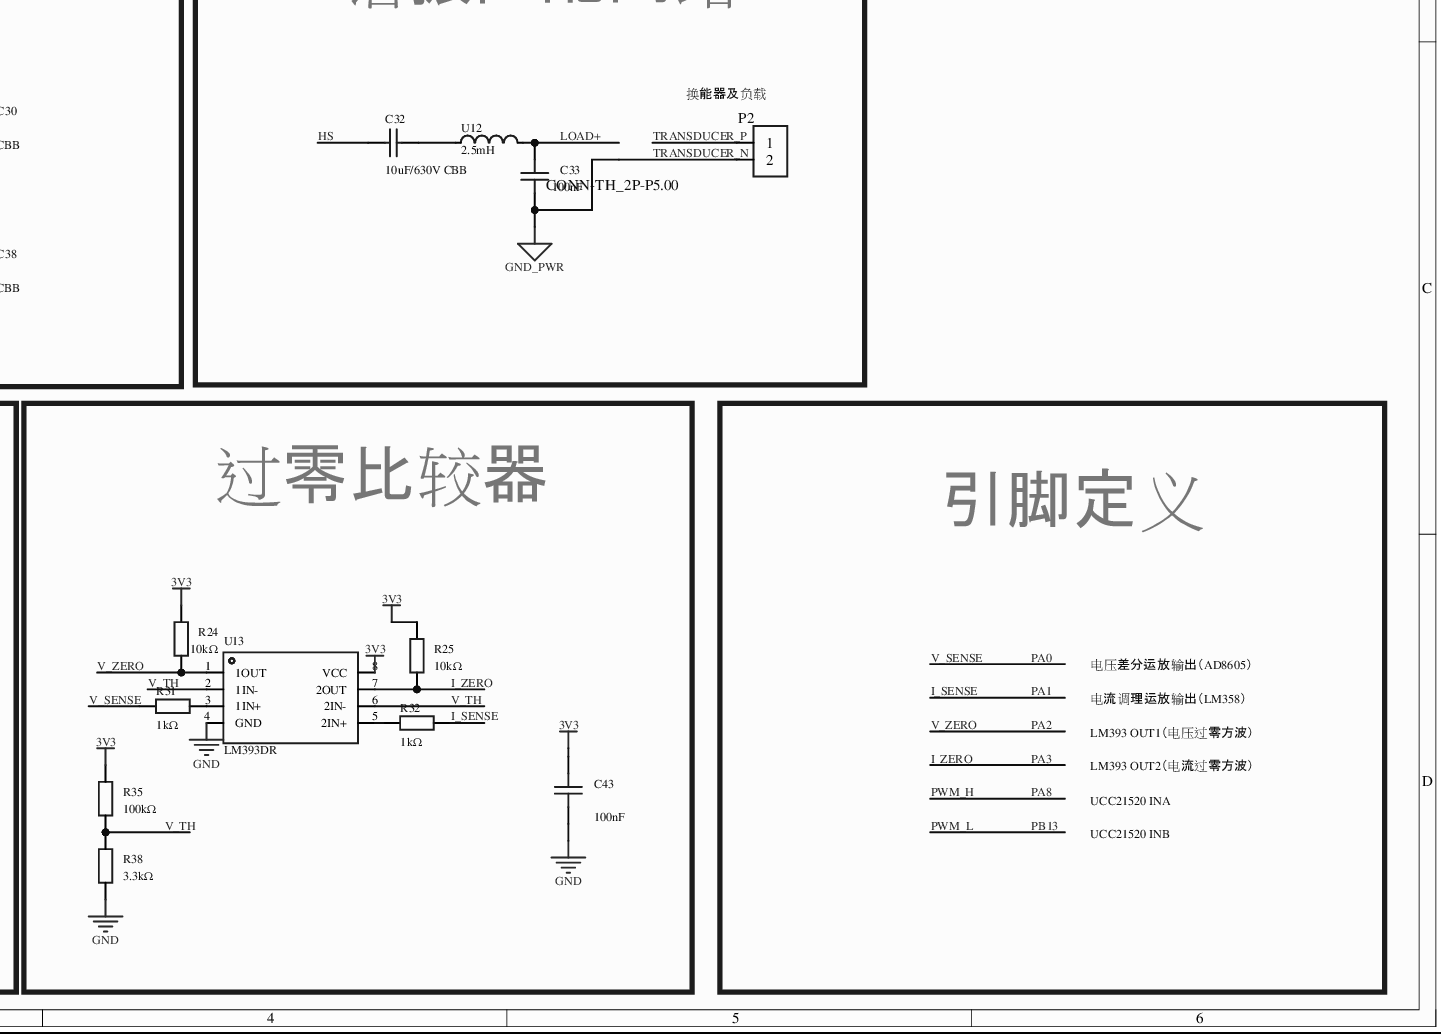
[diagram p0: MISC51807-3.schdoc, bottom right]
# Altium project MISC51807-2.PrjPcb (part 2 of 2)
## Sheet MISC51807-3.schdoc (continued)
### Library data of the parts (continued)
D2 = BYV26C: 二极管配置:独立式;正向压降(Vf):2.5V@1A;直流反向耐压(Vr):600V;整流电流:1A;反向恢复时间(Trr):30ns;; Manufacturer: LGE(鲁光); Symbol: BYV26C_C2903806; AddInBom: yes; ModelId: 24566a456941402eb024cf45acdcf6880819f05c4eef4c71ace90d822a990e87; ModelTransform: 385.826,102.71814,0,0,0,0,0,0,-196.85; Diode Configuration: 独立式; Voltage - DC Reverse(Vr): 600V; Current - Rectified: 1A; Reverse Leakage Current (Ir): 5uA@600V; Reverse Recovery Time (trr): 30ns; Operating Junction Temperature Range: -55℃~+150℃@(Tj); Non-Repetitive Peak Forward Surge Current: 30A; Device: BYV26C; LCSC Part Name: 耐压:600V 电流:1A 反向恢复时间：30ns; SupplierPart: C2903806; ManufacturerPart: BYV26C; Supplier Footprint: DO-41; JLCPCB Part Class: Extended Part; Datasheet: https://item.szlcsc.com/datasheet/BYV26C/3160571.html; Supplier: LCSC; ConvertToPcb: yes; FootprintName: DO-41_BD2.6-L5.1-P9.00-D0.8-RD; ModelName: DO-41_BD2.6-L5.1-P9.00-D0.8-RD; Voltage - Forward(Vf@If): 2.5V@1A
D3 = SR5100_C784810: 二极管配置:独立式;正向压降(Vf):850mV@5A;直流反向耐压(Vr):100V;整流电流:5A;; Manufacturer: FUXINSEMI(富芯森美); 3D Model: f76203e12ec84be0b89e1bb5efd9c700; 3D Model Transform: 582.676,208.5295,0,0,0,0,0,0,-137.795; Diode Configuration: 独立式; Voltage - DC Reverse(Vr): 100V; Current - Rectified: 5A; AddInBom: yes; ModelName: DO-201AD_D5.3-L8.4-P13.6; Symbol: SR5100_C784810; Device: SR5100_C784810; LCSC Part Name: 电压:100V 电流:5A; Supplier Part: C784810; Manufacturer Part: SR5100; Supplier Footprint: DO-27; JLCPCB Part Class: 扩展库; Datasheet: https://atta.szlcsc.com/upload/public/pdf/source/20200917/C784810_F194D3227990C9BBD8D528E4C494EB0B.pdf; Supplier: LCSC; Voltage - Forward(Vf@If): 850mV@5A; Reverse Leakage Current (Ir): -; ConvertToPcb: yes; FootprintName: DO-201AD_BD5.3-L8.4-P12.50-D1.4-RD
D4 D5 = 1N5819_C110032: 正向压降(Vf):550mV@1A;直流反向耐压(Vr):40V;整流电流:1A;; Manufacturer: ST(意法半导体); 3D Model: 6de1e9b71a0d4751b4e9df530304c1a3; 3D Model Transform: 374.015,94.428,0,180,0,0,0,0,-137.795; Reverse Voltage (Vr): 40V; Rectified Current: 1A; Reverse Leakage Current (Ir): 500uA@40V; AddInBom: yes; ModelName: DO-41_D2.4-L4.7-P8.70; Symbol: 1N5819; Device: 1N5819_C110032; LCSC Part Name: 电压:40V 电流:1A; Supplier Part: C110032; Manufacturer Part: 1N5819; Supplier Footprint: DO-41; JLCPCB Part Class: 扩展库; Datasheet: https://atta.szlcsc.com/upload/public/pdf/source/20170428/1493376792224.pdf; Supplier: LCSC; Forward Voltage (Vf@If): 550mV@1A; ConvertToPcb: yes; FootprintName: DO-41_BD2.4-L4.7-P8.70-D0.9-FD
D6 D7 = BZT52C3V3S_C19077437: 二极管配置:独立式;稳压值(标称值):3.3V;稳压值(范围):3.1V~3.5V;耗散功率(Pd):200mW;; Manufacturer: R+O(宏嘉诚); AddInBom: yes; ModelId: 8f7582057468434a979d3a4d6e318d8a0819f05c4eef4c71ace90d822a990e87; ModelTransform: 100.394,49.2125,0,0,0,0,0,0,0; Diode Configuration: 独立式; Zener Voltage(Nom): 3.3V; Reverse Leakage Current (Ir): 5uA@1.0V; Pd - Power Dissipation: 200mW; Impedance(Zzt): 95Ω; Impedance(Zzk): 600Ω; Operating Junction Temperature Range: -55℃~+150℃; Symbol: BZT52C3V3S_C19077437; Device: BZT52C3V3S_C19077437; LCSC Part Name: 表面贴装齐纳二极管; SupplierPart: C19077437; ManufacturerPart: BZT52C3V3S; Supplier Footprint: SOD-323; JLCPCB Part Class: Extended Part; Datasheet: https://item.szlcsc.com/datasheet/BZT52C3V3S/20275522.html; Supplier: LCSC; ConvertToPcb: yes; FootprintName: SOD-323_L1.7-W1.3-LS2.6-RD; ModelName: SOD-323_L1.7-W1.3-LS2.6-RD; Zener Voltage(Range): 3.1V~3.5V
F1 = MTS1315A: 类型:方形保险丝;额定电流:3.15A;额定电压:250V;分断能力:35A@250VAC;; Manufacturer: Reomax(瑞迈); AddInBom: yes; ModelId: 221481fd52dd4abc8b2b4285dcb66f990819f05c4eef4c71ace90d822a990e87; ModelTransform: 330.708,157.48,0,0,0,0,0,0,-157.48; Type: 方形保险丝; Current Rating: 3.15A; Voltage Rating (DC): 250V; Melting I2t: 64; Pitch: 5.08mm; Symbol: MTS1315A; Device: MTS1315A; LCSC Part Name: 方形直插 慢断 250V 3.15A 保险丝; SupplierPart: C2762408; ManufacturerPart: MTS1315A; Supplier Footprint: 插件,P=5.08mm; JLCPCB Part Class: Extended Part; Datasheet: https://item.szlcsc.com/datasheet/MTS1315A/2889364.html; Supplier: LCSC; ConvertToPcb: yes; FootprintName: FUSE-TH_L8.4-W4.0-P5.08-D0.6; ModelName: FUSE-TH_L8.4-W4.0-P5.08-D0.6; Operating Temperature: -55℃~+125℃; Interrupt Rating: 35A@250VAC; Length: 8.4mm; Width: 4mm; Height: 7.2mm
H1 = PZ254V-11-01P: 插针结构:1x1P;间距:2.54mm;行距:-;圆针/方针:方针;安装方式:直插;排数:单排;总PIN位数:1P;额定电流:-;额定电压:-;配合针长度:6mm;塑高:2.5mm;端接针长度:3mm;触头材质:黄铜;触头镀层:-;工作温度:-40℃~+105℃;颜色:黑色;; Manufacturer: XFCN(兴飞); 3D Model: efa57846279b44bfa0a28253a2c74e33; 3D Model Transform: 100,100,0,0,0,0,0,0,-118.11; Pin Structure: 1x1P; Pitch: 2.54mm; Circluar Pins/Square Pins: 方针; AddInBom: yes; ModelName: HDR2.54-M-LI-1X1P; Symbol: PZ254V-11-01P; Device: PZ254V-11-01P; LCSC Part Name: 1x1P 间距:2.54mm 方针 直插; Supplier Part: C492400; Manufacturer Part: PZ254V-11-01P; Supplier Footprint: 插件,P=2.54mm; JLCPCB Part Class: 扩展库; Datasheet: https://atta.szlcsc.com/upload/public/pdf/source/20200309/C492400_46876A5B545F5AE6B8D4A09C46E276E8.pdf; Supplier: LCSC; Row Spacing: -; Mounting Type: 直插; Number of Rows: 单排; Number of Pins: 1P; Current Rating: -; Voltage Rating (Max): -; Length of Mating Pin: 6mm; Insulation Height: 2.5mm; Length of End Connection Pin: 3mm; Contact Material: 黄铜; Contact Plating: -; Operating Temperature: -40℃~+105℃; Color: 黑色; ConvertToPcb: yes; FootprintName: HDR-TH_1P-P2.54-V-M
J1 J2 = 2.54-1*20P直针: 排数:单排;总PIN位数:20;间距:2.54mm;插针结构:1x20P;行距:-;安装类型:直插;圆针/方针:方针;额定电流:3A;额定电压:-;配合针长度:-;塑高:-;端接针长度:-;触头材质:黄铜;触头镀层:-;工作温度范围:-40~+105;颜色:黑色;; Manufacturer: BOOMELE(博穆精密); Symbol: Header-Male-2.54_1x20; 3D Model: f68709be121d406db68b06f32a595389; 3D Model Transform: 1999.996,100,0,0,0,0,0,2.48,-118.11; Pitch: 2.54mm; Pin Structure: 1x20P; Circluar Pins/Square Pins: 方针; Current Rating (Max): 3A; AddInBom: yes; ModelName: HDR-M-2.54_1x20; Device: 2.54-1*20P直针; Operating Temperature Range: -40~+105; LCSC Part Name: 2.54mm 1x20P 直插 方针; Supplier Part: C50981; Manufacturer Part: 2.54-1*20P直针; Supplier Footprint: 插件,P=2.54mm; JLCPCB Part Class: Extended Part; Datasheet: https://atta.szlcsc.com/upload/public/pdf/source/20151109/1457707571495.pdf; Supplier: LCSC; Number of Rows: 单排; Number of Pins: 20; Row Spacing: -; Mounting Type: 直插; Voltage Rating (Max): -; Length of Mating Pin: -; Insulation Height: -; Length of End Connection Pin: -; Contact Material: 黄铜; Contact Plating: -; Color: 黑色; ConvertToPcb: yes; FootprintName: HDR-TH_20P-P2.54-V-M-1
L1 = PDMCAT16128-103ML: 通道数:2;电感@频率:10mH@1kHz;直流电阻(DCR):75mΩ;; Manufacturer: PROD(谱罗德); AddInBom: yes; ModelId: 59532b68e412455698164cb9480e4efc0819f05c4eef4c71ace90d822a990e87; ModelTransform: 787.4,444.881,0,0,0,0,-0.591,0,-196.85; Number of Lines: 2; Voltage Withstand: 600V@AC,3secs; Current Rating: 3A; Voltage Rating - DC: 600V; DC Resistance(DCR): 75mΩ; Symbol: PDMCAT16128-103ML; Device: PDMCAT16128-103ML; LCSC Part Name: 两路 插件共模滤波器; SupplierPart: C2762380; ManufacturerPart: PDMCAT16128-103ML; Supplier Footprint: 插件,20x18mm; JLCPCB Part Class: Extended Part; Datasheet: https://atta.szlcsc.com/upload/public/pdf/source/20210322/C2762380_4CF5A8B18369ADCA8640E34A9EF957E4.pdf; Supplier: LCSC; ConvertToPcb: yes; FootprintName: IND-TH_4P-L20.0-W12.0-P6.00-LS10.0-BL; ModelName: IND-TH_4P-L20.0-W12.0-P6.00-LS10.0-BL; Inductance @ Frequency: 10mH@1kHz; Voltage Rating (AC): 600V; Operating Temperature: -25℃~+85℃
L2 = SLP0810R-102MTT: 电感值:1mH;精度:±20%;额定电流:500mA;类型:工字电感;; Manufacturer: Sunltech(顺磁); AddInBom: yes; ModelId: f824c3cd5f0947e0ad34b4cb921321ba0819f05c4eef4c71ace90d822a990e87; ModelName: IND-TH_BD8.5-H8.3-P5.00-D0.6; ModelTransform: 334.645,334.645,0,0,0,0,-0.005,0,-196.85; Tolerance: ±20%; Current Rating: 500mA; DC Resistance(DCR): 1.8Ω; Type: 工字电感; Symbol: SLP0810R-102MTT; Device: SLP0810R-102MTT; LCSC Part Name: 1mH ±20%; SupplierPart: C364093; ManufacturerPart: SLP0810R-102MTT; Supplier Footprint: 插件,D8.5xL12mm; JLCPCB Part Class: Extended Part; Datasheet: https://item.szlcsc.com/datasheet/SLP0810R-102MTT/338381.html; Supplier: LCSC; ConvertToPcb: yes; FootprintName: IND-TH_BD8.5-P5.00-D0.6; Value: 1mH
OLED1 = 0.96OLED模块_4P: 3D Model: 79c000fdb68d45a296c2e9bedf4f9055; 3D Model Transform: 1393.69792,1318.895,0,0,0,0,0,-560.079,-137.795; ConvertToPcb: yes; Symbol: 0.96OLED模块_4P; Device: 0.96OLED模块_4P; Supplier Footprint: 插件; AddInBom: yes; FootprintName: 0.96OLED_4P; ModelName: 0.96OLED_4P
P1 P2 = CONN-TH_2P-P5.00: Add into BOM: yes; 3D Model: 82ed0e208d9a4cc2ac854dcad4b56f25; Symbol: CONN-TH_2P-P5.00; Device: CONN-TH_2P-P5.00; Convert to PCB: yes; Supplier: LCSC; FootprintName: CONN-TH_2P-P5.00; ModelName: CONN-TH_2P-P5.00
Q1 Q2 = IRF840_C2980294: 数量:1个N沟道;漏源电压(Vdss):500V;连续漏极电流(Id):8A;导通电阻(RDS(on)):730mΩ@10V;耗散功率(Pd):134W;阈值电压(Vgs(th)):3V@250uA;; Manufacturer: minos(迈诺斯); AddInBom: yes; ModelId: 0369bc25c9bd44718af72a1d71ffd3cd0819f05c4eef4c71ace90d822a990e87; ModelTransform: 401.574,177.204,0,0,0,0,0,24.606,-196.85; Number: 1个N沟道; Drain to Source Voltage: 500V; Current - Continuous Drain(Id): 8A; Pd - Power Dissipation: 134W; Gate Charge(Qg): 25nC@10V; Input Capacitance(Ciss): 1.57nF; Reverse Transfer Capacitance (Crss@Vds): 20pF; Type: N沟道; Output Capacitance(Coss): 195pF; Symbol: IRF840_C2980294; Device: IRF840_C2980294; LCSC Part Name: N沟道,电流:8A,耐压:500V; SupplierPart: C2980294; ManufacturerPart: IRF840; Supplier Footprint: TO-220; JLCPCB Part Class: Extended Part; Datasheet: https://item.szlcsc.com/datasheet/IRF840/3401452.html; Supplier: LCSC; ConvertToPcb: yes; FootprintName: TO-220-3_L10.2-W4.5-P2.54-L-1; ModelName: TO-220-3_L10.2-W4.5-P2.54-L-1; RDS(on): 730mΩ@10V; Gate Threshold Voltage (Vgs(th)): 3V@250uA; Operating Temperature: -
R1 = 0603WAF6201T5E: 电阻类型:厚膜电阻;阻值:6.2kΩ;精度:±1%;功率:100mW;工作电压:75V;温度系数:±100ppm/℃;; Manufacturer: UNI-ROYAL(厚声); AddInBom: yes; ModelId: fc143cca1e79419f9cd78b61e9279f080819f05c4eef4c71ace90d822a990e87; ModelTransform: 31.8897,63.7794,0,90,0,0,0,0,0; Tolerance: ±1%; Power(Watts): 100mW; Voltage-Supply(Max): 75V; Symbol: 0603WAF6201T5E; Device: 0603WAF6201T5E; LCSC Part Name: 6.2kΩ ±1% 100mW 厚膜电阻; SupplierPart: C4260; ManufacturerPart: 0603WAF6201T5E; Supplier Footprint: 0603; JLCPCB Part Class: Basic Part; Datasheet: https://item.szlcsc.com/datasheet/0603WAF6201T5E/4667.html; Supplier: LCSC; ConvertToPcb: yes; FootprintName: R0603; ModelName: R0603; Type: 厚膜电阻; Value: 6.2kΩ; Temperature Coefficient: ±100ppm/℃; Operating Temperature: -55℃~+155℃
R2 = 0603WAF2002T5E: 电阻类型:厚膜电阻;阻值:20kΩ;精度:±1%;功率:100mW;工作电压:75V;温度系数:±100ppm/℃;; Manufacturer: UNI-ROYAL(厚声); AddInBom: yes; ModelId: fc143cca1e79419f9cd78b61e9279f080819f05c4eef4c71ace90d822a990e87; ModelTransform: 31.8897,63.7794,0,90,0,0,0,0,0; Tolerance: ±1%; Power(Watts): 100mW; Voltage-Supply(Max): 75V; Symbol: 0603WAF2002T5E; Device: 0603WAF2002T5E; LCSC Part Name: 20kΩ ±1% 100mW 厚膜电阻; SupplierPart: C4184; ManufacturerPart: 0603WAF2002T5E; Supplier Footprint: 0603; JLCPCB Part Class: Basic Part; Datasheet: https://item.szlcsc.com/datasheet/0603WAF2002T5E/4591.html; Supplier: LCSC; ConvertToPcb: yes; FootprintName: R0603; ModelName: R0603; Type: 厚膜电阻; Value: 20kΩ; Temperature Coefficient: ±100ppm/℃; Operating Temperature: -55℃~+155℃
R3 = 14D471K_C49069733: 压敏电压:470V;钳位电压:775V;工作电压(DC):385V;工作电压(AC):300V;; Manufacturer: R+O(宏嘉诚); AddInBom: yes; ModelId: 3cca2a1a348a43d9bb99ecdc91f351c80819f05c4eef4c71ace90d822a990e87; ModelName: RES-TH_L15.5-W5.6-H18.5-P7.50-D0.8-S1.90; ModelTransform: 610.19083,220.472,0,0,0,0,0,0,-196.85; Varistor Voltage: 470V; Clamping Voltage: 775V; Maximum DC Volts: 385V; Maximum AC Volts: 300V; Peak Current: 4.5kA; Energy: 148J; Rated Wattage: 600mW; Symbol: 14D471K_C49069733; Device: 14D471K_C49069733; LCSC Part Name: 775V 148J; SupplierPart: C49069733; ManufacturerPart: 14D471K; Supplier Footprint: 插件,P=7.5mm; JLCPCB Part Class: Extended Part; Datasheet: https://item.szlcsc.com/datasheet/14D471K/51445299.html; Supplier: LCSC; ConvertToPcb: yes; FootprintName: RES-TH_L15.5-W5.6-P7.50-D0.8-S1.90; Value: 420pF@1kHz
R4 = FMP200JR-52-220K: 电阻类型:金属膜电阻;阻值:220kΩ;精度:±5%;功率:2W;温度系数:±100ppm/℃;; Manufacturer: YAGEO(国巨); AddInBom: yes; ModelId: 8ab905774ec2447d84fda7276baf35870819f05c4eef4c71ace90d822a990e87; ModelTransform: 543.306,153.44056,0,0,0,0,0,0,-196.85; Tolerance: ±5%; Power(Watts): 2W; Symbol: FMP200JR-52-220K; Device: FMP200JR-52-220K; LCSC Part Name: 金属膜电阻 220kΩ ±5% 2W; SupplierPart: C1759543; ManufacturerPart: FMP200JR-52-220K; Supplier Footprint: 插件,D3.9xL9mm; JLCPCB Part Class: Extended Part; Datasheet: https://item.szlcsc.com/datasheet/FMP200JR-52-220K/1850325.html; Supplier: LCSC; ConvertToPcb: yes; FootprintName: RES-TH_BD3.9-L9.0-P13.00-D0.8; ModelName: RES-TH_BD3.9-L9.0-P13.00-D0.8; Type: 金属膜电阻; Value: 220kΩ; Temperature Coefficient: ±100ppm/℃; Operating Temperature: -55℃~+155℃
R6 R7 = 0603WAF1002T5E: 电阻类型:厚膜电阻;阻值:10kΩ;精度:±1%;功率:100mW;温度系数:±100ppm/;最大工作电压:75V;工作温度范围:-55~+155;; Manufacturer: UNI-ROYAL(厚声); 3D Model: 3281a289d46d4bb1877be1eabd090e13; 3D Model Transform: 62.992,31.496,0,0,0,0,0,0,0; Tolerance: ±1%; Power(Watts): 100mW; Overload Voltage (Max): 75V; AddInBom: yes; ModelName: R0603_L1.6-W0.8-H0.8; Symbol: 0603WAF1002T5E; Device: 0603WAF1002T5E; Value: 10kΩ; Temperature Coefficient: ±100ppm/; Operating Temperature Range: -55~+155; LCSC Part Name: 10kΩ ±1% 100mW; Supplier Part: C25804; Manufacturer Part: 0603WAF1002T5E; Supplier Footprint: 0603; JLCPCB Part Class: Basic Part; Datasheet: https://atta.szlcsc.com/upload/public/pdf/source/20200306/C422600_1E6D84923E4A46A82E41ADD87F860B5C.pdf; Supplier: LCSC; Type: 厚膜电阻; ConvertToPcb: yes; FootprintName: R0603_1
R8 R9 = 0603WAF4701T5E: 电阻类型:厚膜电阻;阻值:4.7kΩ;精度:±1%;功率:100mW;工作电压:75V;温度系数:±100ppm/℃;; Manufacturer: UNI-ROYAL(厚声); AddInBom: yes; ModelId: fc143cca1e79419f9cd78b61e9279f080819f05c4eef4c71ace90d822a990e87; ModelTransform: 31.8897,63.7794,0,90,0,0,0,0,0; Tolerance: ±1%; Power(Watts): 100mW; Voltage-Supply(Max): 75V; Symbol: 0603WAF4701T5E; Device: 0603WAF4701T5E; LCSC Part Name: 4.7kΩ ±1% 100mW 厚膜电阻; SupplierPart: C23162; ManufacturerPart: 0603WAF4701T5E; Supplier Footprint: 0603; JLCPCB Part Class: Basic Part; Datasheet: https://item.szlcsc.com/datasheet/0603WAF4701T5E/23889.html; Supplier: LCSC; ConvertToPcb: yes; FootprintName: R0603; ModelName: R0603; Type: 厚膜电阻; Value: 4.7kΩ; Temperature Coefficient: ±100ppm/℃; Operating Temperature: -55℃~+155℃
R11-R21 = Res_0805: Symbol: 电阻; 3D Model: 37a81e68749a4138bd2dfa6897b24b85; 3D Model Transform: 78.74,51.181,0,0,0,0,0,-0.0005,0; ConvertToPcb: yes; ModelName: R0805_L2.0-W1.3-H0.6; Device: Res_0805; Supplier Footprint: 0805; AddInBom: yes; FootprintName: R0805
  R11 R12 R17: Value: 4.7R
  R13 R14: Value: 47R
  R15 R20: Value: 10r
  R16 R18 R21: Value: 10K
  R19: Value: 4.7k
R22-R25 R28 R33 R36 R37 = 0805W8F1002T5E_C17414: 电阻类型:厚膜电阻;阻值:10kΩ;精度:±1%;功率:125mW;工作电压:150V;温度系数:±100ppm/℃;; Manufacturer: UNI-ROYAL(厚声); AddInBom: yes; ModelId: 37a81e68749a4138bd2dfa6897b24b850819f05c4eef4c71ace90d822a990e87; ModelName: R0805_L2.0-W1.3-H0.6; ModelTransform: 78.74,51.181,0,0,0,0,0,-0.0005,0; Tolerance: ±1%; Power(Watts): 125mW; Voltage-Supply(Max): 150V; Symbol: 0805W8F1002T5E; Device: 0805W8F1002T5E_C17414; LCSC Part Name: 10kΩ ±1% 125mW 厚膜电阻; SupplierPart: C17414; ManufacturerPart: 0805W8F1002T5E; Supplier Footprint: 0805; JLCPCB Part Class: Basic Part; Datasheet: https://item.szlcsc.com/datasheet/0805W8F1002T5E/18102.html; Supplier: LCSC; ConvertToPcb: yes; FootprintName: R0805; Type: 厚膜电阻; Value: 10kΩ; Temperature Coefficient: ±100ppm/℃; Operating Temperature: -55℃~+155℃
R26 R30 = 1206W4F1004T5E: 电阻类型:厚膜电阻;阻值:1MΩ;精度:±1%;功率:250mW;工作电压:200V;温度系数:±100ppm/℃;; Manufacturer: UNI-ROYAL(厚声); AddInBom: yes; ModelId: 89a1f13db2384da588040e0b3c55bf660819f05c4eef4c71ace90d822a990e87; ModelName: R1206_L3.2-W1.6-H0.6; ModelTransform: 125.984,62.992,0,0,0,0,0,0,0; Tolerance: ±1%; Power(Watts): 250mW; Voltage-Supply(Max): 200V; Symbol: 1206W4F1004T5E; Device: 1206W4F1004T5E; LCSC Part Name: 1MΩ ±1% 250mW 厚膜电阻; SupplierPart: C17927; ManufacturerPart: 1206W4F1004T5E; Supplier Footprint: 1206; JLCPCB Part Class: Basic Part; Datasheet: https://item.szlcsc.com/datasheet/1206W4F1004T5E/18615.html; Supplier: LCSC; ConvertToPcb: yes; FootprintName: R1206; Type: 厚膜电阻; Value: 1MΩ; Temperature Coefficient: ±100ppm/℃; Operating Temperature: -55℃~+155℃
R27 R34 = 0805W8F1000T5E: 电阻类型:厚膜电阻;阻值:100Ω;精度:±1%;功率:125mW;最大工作电压:150V;温度系数:±100ppm/℃;; Manufacturer: UNI-ROYAL(厚声); AddInBom: yes; ModelId: 37a81e68749a4138bd2dfa6897b24b850819f05c4eef4c71ace90d822a990e87; ModelName: R0805_L2.0-W1.3-H0.6; ModelTransform: 78.74,51.181,0,0,0,0,0,-0.0005,0; Tolerance: ±1%; Power(Watts): 125mW; Overload Voltage (Max): 150V; Symbol: 0805W8F1000T5E; Device: 0805W8F1000T5E; LCSC Part Name: 100Ω ±1% 125mW 厚膜电阻; SupplierPart: C17408; ManufacturerPart: 0805W8F1000T5E; Supplier Footprint: 0805; JLCPCB Part Class: Basic Part; Datasheet: https://atta.szlcsc.com/upload/public/pdf/source/20200306/C422600_1E6D84923E4A46A82E41ADD87F860B5C.pdf; Supplier: LCSC; ConvertToPcb: yes; FootprintName: R0805; Type: 厚膜电阻; Value: 100Ω; Temperature Coefficient: ±100ppm/℃; Operating Temperature Range: -55℃~+155℃
R29 = FRC0805J821 TS: 电阻类型:厚膜电阻;阻值:820Ω;精度:±5%;功率:125mW;工作电压:150V;温度系数:±100ppm/℃;; Manufacturer: FOJAN(富捷); AddInBom: yes; ModelId: 37a81e68749a4138bd2dfa6897b24b8554bc6f14d6c140e19f9d5807e5437d2c; ModelName: R0805_L2.0-W1.3-H0.6; ModelTransform: 78.74,51.181,0,0,0,0,0,-0.0005,0; Tolerance: ±5%; Power(Watts): 125mW; Voltage-Supply(Max): 150V; Symbol: FRC0805J821 TS; Device: FRC0805J821 TS; LCSC Part Name: 820Ω ±5% 125mW 厚膜电阻; SupplierPart: C2933571; ManufacturerPart: FRC0805J821 TS; Supplier Footprint: 0805; JLCPCB Part Class: 扩展库; Datasheet: https://item.szlcsc.com/datasheet/FRC0805J821%2520TS/3279673.html; Supplier: LCSC; ConvertToPcb: yes; Type: 厚膜电阻; Value: 820Ω; Temperature Coefficient: ±100ppm/℃; Operating Temperature: -55℃~+155℃; FootprintName: R0805
R31 R32 = 1kΩ: Manufacturer: UNI-ROYAL(厚声); Symbol: 0603WAF1001T5E; AddInBom: yes; Tolerance: ±1%; Power(Watts): 100mW; Overload Voltage (Max): 75V; Temperature Coefficient: ±100ppm/℃; ModelId: fc143cca1e79419f9cd78b61e9279f087eafdc8b457f47c5b4ec02ac0140f89b; Device: 1kΩ; LCSC Part Name: 1kΩ ±1% 100mW 厚膜电阻; SupplierPart: C21190; ManufacturerPart: 0603WAF1001T5E; Supplier Footprint: 0603; JLCPCB Part Class: 基础库; Datasheet: https://atta.szlcsc.com/upload/public/pdf/source/20200306/C422600_1E6D84923E4A46A82E41ADD87F860B5C.pdf; Supplier: LCSC; ConvertToPcb: yes; Type: 厚膜电阻; Value: 1kΩ; Operating Temperature Range: -55℃~+155℃; FootprintName: R0603; ModelName: R0603
R35 = 100kΩ: Manufacturer: YAGEO(国巨); ManufacturerPart: RC0603FR-07100KL; ConvertToPcb: yes; ModelId: fc143cca1e79419f9cd78b61e9279f0857dedad79084406cbdf9ff24654f194a; Symbol: 100kΩ; Device: 100kΩ; Supplier: LCSC; SupplierPart: C14675; JLCPCB Part Class: Extended Part; AddInBom: yes; FootprintName: R0603; ModelName: R0603
R38 = 0603WAF3301T5E: 阻值:3.3kΩ;精度:±1%;温度系数:±100ppm/℃;功率:1/10W;最大工作电压:75V;工作温度范围:-55℃~+155℃;; Manufacturer: UNI-ROYAL(厚声); AddInBom: yes; ModelId: 3281a289d46d4bb1877be1eabd090e1300b5e15d11014781ab595edbebbd87c6; ModelName: R0603_L1.6-W0.8-H0.8; ModelTransform: 62.992,31.496,0,0,0,0,0,0,0; Tolerance: ±1%; Power(Watts): 1/10W; Overload Voltage (Max): 75V; Symbol: 0603WAF3301T5E; Device: 0603WAF3301T5E; ConvertToPcb: yes; LCSC Part Name: 3.3KΩ ±1%; SupplierPart: C22978; ManufacturerPart: 0603WAF3301T5E; Supplier Footprint: 0603; JLCPCB Part Class: Basic Part; Datasheet: https://atta.szlcsc.com/upload/public/pdf/source/20170920/C22978_1505901014515982365.pdf; Supplier: LCSC; Value: 3.3kΩ; Temperature Coefficient: ±100ppm/℃; Operating Temperature Range: -55℃~+155℃; FootprintName: R0603_NEW
SW2 SW3 = TS-1088-AR02016: 触点电流:50mA;额定电压(DC):12V;绝缘电阻:100MΩ;电路结构:单刀单掷;安装方式:立贴;作用力:160gf@±50gf;机械寿命:10万次;带支架:否;; Manufacturer: XUNPU(讯普); Add into BOM: yes; 3D Model: b26698b69f274ffabef8a26c7d0e5dd1; 3D Model Transform: 188.976,114.174,0,0,0,0,0,0,0; Contact Current: 50mA; Voltage Rating (DC): 12V; Insulation Resistance: 100MΩ; Circuit: 单刀单掷; Actuator Style: 圆形按钮; Actuator/Cap Color: 黑色; Mechanical Life: 10万次; Pin Style: SMD接片; Switch Length: 4mm; Switch Width: 3mm; Switch Height: 2mm; Strike Gundam: 否; ModelName: SW-SMD_L3.9-W2.9-H2.0-LS4.8; Symbol: TS-1088-AR02016; Device: TS-1088-AR02016; Convert to PCB: yes; LCSC Part Name: 4*3*2mm 立贴 轻触开关; Supplier Part: C720477; Manufacturer Part: TS-1088-AR02016; Supplier Footprint: SMD; JLCPCB Part Class: 扩展库; Datasheet: https://atta.szlcsc.com/upload/public/pdf/source/20200810/C720475_60D09DD6C54279ADDB2DC25100F1CC11.pdf; Supplier: LCSC; Mounting Style: 立贴; Operating Force: 160gf@±50gf; Operating Temperature: -30℃~+80℃; FootprintName: SW-SMD_L3.9-W3.0-P4.45
T1 = TA-1005M: ConvertToPcb: yes; Symbol: TA-1005M; Device: TA-1005M; AddInBom: yes; FootprintName: TA-1005M
U1 = CC1H103ZA1ED3F4D1100: 容值:10nF;精度:-20%~+80%;额定电压:50V;温度系数:Y5V;; Manufacturer: Dersonic(德尔创); AddInBom: yes; ModelId: 2000e098e2ac4561b8c8a10584815b3a0819f05c4eef4c71ace90d822a990e87; ModelTransform: 217.59145,98.425,0,0,0,0,0,0,-196.85; Voltage Rating: 50V; Pin Spacing: 2.54mm; Temperature Coefficient: Y5V; Body Thickness: 2.4mm; Symbol: CC1H103ZA1ED3F4D1100; Device: CC1H103ZA1ED3F4D1100; LCSC Part Name: 10nF -20%~+80% 50V; SupplierPart: C2832505; ManufacturerPart: CC1H103ZA1ED3F4D1100; Supplier Footprint: 插件,P=2.54mm; JLCPCB Part Class: Extended Part; Datasheet: https://item.szlcsc.com/datasheet/CC1H103ZA1ED3F4D1100/2990643.html; Supplier: LCSC; ConvertToPcb: yes; FootprintName: CAP-TH_L5.0-W2.5-P2.50-D0.5; ModelName: CAP-TH_L5.0-W2.5-P2.50-D0.5; Value: 10nF; Tolerance: -20%~+80%; Diameter: 5mm
U2 = LM7805_C845394: 输出类型:固定;工作电压:35V;输出电压:5V;输出电流:-;电源纹波抑制比(PSRR):73dB@(120Hz);输出极性:正极;; Manufacturer: TF(拓锋); AddInBom: yes; ModelId: b3c9e38e4428458f8b925050989b538f0819f05c4eef4c71ace90d822a990e87; ModelTransform: 401.574,178.58232,0,0,0,0,0,25.59,-196.85; Output Type: 固定; Voltage - Supply: 35V; Output Voltage: 5V; Voltage Dropout: 2V@(1A); standby current: 5mA; Noise: 42uV; Output Configuration: 正极; Number of Outputs: 1; Symbol: LM7805; Device: LM7805_C845394; LCSC Part Name: LM7805; SupplierPart: C845394; ManufacturerPart: LM7805; Supplier Footprint: TO-220; JLCPCB Part Class: Extended Part; Datasheet: https://item.szlcsc.com/datasheet/LM7805/905247.html; Supplier: LCSC; ConvertToPcb: yes; FootprintName: TO-220-3_L10.0-W4.5-P2.54-L; ModelName: TO-220-3_L10.0-W4.5-P2.54-L; Output Current: -; Power Supply Rejection Ratio (PSRR): 73dB@(120Hz); Operating Temperature: 0℃~+150℃@(Tj)
U3 = B1205S-1WR3_C5365649: B1205S-1WR3小体积，高效率的微小功率,定电压输入,隔离非稳压单路输出,DC/DC模块电源；该系列产品是专门针对板上电源系统中需要产生一组与输入电源隔离的电压的应用场合而设计的。该产品适用于：1)输入电源的电压比较稳定（电压变化范围±10%Vin）;2)输入输出之间要求隔离（隔离电压≤1500VDC）；3)对输出电压稳定度要求不高；4)典型应用：纯数字电路场合，一般低频模拟电路场合，继电器驱动电路，数据交换电路场合等;; Manufacturer: YLPTEC(易川); AddInBom: yes; ModelId: 8bab021673d24e22b9d4c82ca7eecfe90819f05c4eef4c71ace90d822a990e87; ModelTransform: 452.755,236.614,0,0,0,0,0,90.551,-157.48; Number of Channels: 1; Output Power: 1W; Voltage - Supply: 10.8V~13.2V; Conversion Efficiency: 88%; Output Voltage: 5V; Output Current(Max): 200mA; Capacitive Load(Max): 2400uF; Isolation Voltage(Vrms): 1.5kV; No-Load Input Current: 8mA; Ripple Noise: 30mVp-p; Symbol: B1205S-1WR3_C5365649; Device: B1205S-1WR3_C5365649; LCSC Part Name: DC-DC转换器; SupplierPart: C5365649; ManufacturerPart: B1205S-1WR3; Supplier Footprint: SIP,11.5x6mm; JLCPCB Part Class: Extended Part; Datasheet: https://item.szlcsc.com/datasheet/B1205S-1WR3/6197779.html; Supplier: LCSC; ConvertToPcb: yes; FootprintName: PWRM-TH_4P-L11.5-W6.0-P2.54_B1503S; ModelName: PWRM-TH_4P-L11.5-W6.0-P2.54_B1503S; Type: 降压型; Features: 短路保护; Operating Temperature: -40℃~+105℃; Value: 260kHz
U4 = LNK304PN: 工作电压:-;开关频率:66kHz;输出电流:170mA;晶体管耐压:700V;; Manufacturer: Power Integrations(帕沃英蒂格盛); AddInBom: yes; ModelId: 5242b41408b548f4a467f19308f6d6490819f05c4eef4c71ace90d822a990e87; ModelName: DIP-8_7P-L9.3-W6.4-H4.6-P2.54-LS7.6-BL-PE6; ModelTransform: 364.173,311.8104,0,0,0,0,0,0,-118.11; Isolation: 非隔离; Frequency - Switching: 66kHz; Output Current: 170mA; Duty Cycle(Max): 69%; Voltage - Breakdown: 700V; Topology: 降压-升压式；反激式；降压式; Output Voltage: 12V; Symbol: LNK304PN; Device: LNK304PN; LCSC Part Name: 700V 170mA; SupplierPart: C23875; ManufacturerPart: LNK304PN; Supplier Footprint: DIP-7; JLCPCB Part Class: Extended Part; Datasheet: https://item.szlcsc.com/datasheet/LNK304PN/24615.html; Supplier: LCSC; ConvertToPcb: yes; FootprintName: DIP-8_7P-L9.7-W6.4-P2.54-LS7.6-BL-PE6; Voltage - Supply: -; Pd - Power Dissipation: -; Features: 过热保护(OTP)；短路保护(SCP)；过流保护(OCP); Operating Temperature: -40℃~+150℃@(Tj); Working Mode: -; Feedback System: -
U5 = AMS1117-3.3_C6186: 输出类型:固定;工作电压:15V;输出电压:3.3V;输出电流:1A;电源纹波抑制比(PSRR):72dB@(120Hz);输出极性:正极;; Manufacturer: AMS; AddInBom: yes; ModelId: 925194bf9823436183a3e0b978a8d0760819f05c4eef4c71ace90d822a990e87; ModelName: SOT-223-4P_L6.5-W3.5-H1.6-LS7.0-P2.30; ModelTransform: 279.89794,255.905,0,180,0,0,-3.9385,-0.0005,0; Output Type: 固定; Voltage - Supply: 15V; Output Voltage: 3.3V; Output Current: 1A; Voltage Dropout: 1.1V@(800mA); standby current: 5mA; Noise: 0.003%Vout; Output Configuration: 正极; Number of Outputs: 1; Symbol: AMS1117-3.3; Device: AMS1117-3.3_C6186; LCSC Part Name: 3.3V 1A 15V; SupplierPart: C6186; ManufacturerPart: AMS1117-3.3; Supplier Footprint: SOT-223; JLCPCB Part Class: Basic Part; Datasheet: https://item.szlcsc.com/datasheet/AMS1117-3.3/6652.html; Supplier: LCSC; ConvertToPcb: yes; FootprintName: SOT-223-3_L6.5-W3.4-P2.30-LS7.0-BR; Power Supply Rejection Ratio (PSRR): 72dB@(120Hz); Features: 过流保护；热关断; Operating Temperature: -40℃~+125℃
U6 U7 = 152EC0566: 容值:470uF;精度:±20%;额定电压:450V;脚间距:-;等效串联电阻(ESR):-;纹波电流:-;; Manufacturer: KNSCHA(科尼盛); AddInBom: yes; ModelId: 282776b5784f4d31a5dc397d413dc0050819f05c4eef4c71ace90d822a990e87; ModelTransform: 1377.918,1377.93406,0,180,0,0,-0.001,0,-216.535; Tolerance: ±20%; Voltage Rating: 450V; Symbol: 152EC0566; Device: 152EC0566; LCSC Part Name: 470uF ±20% 450V; SupplierPart: C20607183; ManufacturerPart: 152EC0566; Supplier Footprint: 插件,D35xL50mm; JLCPCB Part Class: Extended Part; Datasheet: https://item.szlcsc.com/datasheet/152EC0566/21952596.html; Supplier: LCSC; ConvertToPcb: yes; FootprintName: CAP-TH_BD35.0-P10.00-D1.5-FD; ModelName: CAP-TH_BD35.0-P10.00-D1.5-FD; Value: 470uF; Pin Spacing: -; Equivalent Series Resistance(ESR): -; Ripple Current: -; Diameter: 35mm; Height - Seated (Max): 50mm; Lifetime: -; Operating Temperature: -40℃~+105℃
U11 = UCC21520ADWR: Manufacturer: TI(德州仪器); 3D Model: 2da8125c657e49328ba6fa7b098653dd; 3D Model Transform: 405.511,409.68154,0,0,0,0,-0.0005,0,0; Isolation voltage(Vrms): 5700; Number of Channels: 2; Voltage - Supply (Input): 3V~18V; Peak Output Current(source): 4A; Peak Output Current(sink): 6A; Fall Time: 12ns; Propagation Delay tpLH: 45ns; Input Logic Level - High: 1.2V~2V; Input Logic Level - Low: 0.8V~1.2V; Quiescent Current(Iq): 2000uA; CMTI(kV/us): 125kV/us; Voltage - Supply (Driver): 6.5V~25V; AddInBom: yes; ModelName: SOIC-16_L10.3-W7.5-H2.7-LS10.3-P1.27; Symbol: UCC21520ADWR; Device: UCC21520ADWR; LCSC Part Name: UCC21520ADWR; Supplier Part: C2863027; Manufacturer Part: UCC21520ADWR; Supplier Footprint: SOIC-16-300mil; JLCPCB Part Class: 扩展库; Datasheet: https://www.ti.com/cn/lit/gpn/ucc21520; Supplier: LCSC; Operating Temperature: -40℃~+150℃@(Tj); Propagation Delay tpHL: 45ns; ConvertToPcb: yes; FootprintName: SOIC-16_L10.3-W7.5-P1.27-LS10.3-BL
U12 = XR8*10-252K-S: 电感值:2.5mH;精度:±10%;类型:工字电感;; Manufacturer: XR(祥如); AddInBom: yes; ModelId: 05a8e71b894b42c1a2532ee6cc82a5b80819f05c4eef4c71ace90d822a990e87; ModelName: IND-TH_BD9.5-H12.5-P5.00-D0.7; ModelTransform: 374.015,372.969,0,90,0,0,-0.005,0,-196.85; Tolerance: ±10%; DC Resistance(DCR): 3.7Ω; Wire Diameter: 0.18mm; Symbol: XR8*10-252K-S; Device: XR8*10-252K-S; LCSC Part Name: 2.5mH ±10% 工字电感; SupplierPart: C5358112; ManufacturerPart: XR8*10-252K-S; Supplier Footprint: 插件,D8xL10mm; JLCPCB Part Class: Extended Part; Datasheet: https://item.szlcsc.com/datasheet/XR8*10-252K-S/6167538.html; Supplier: LCSC; ConvertToPcb: yes; FootprintName: IND-TH_BD9.5-P5.00-D0.7; Value: 2.5mH; Type: 工字电感
U13 = LM393DR: 比较器数:双路;输入失调电压(Vos):2mV;输入偏置电流(Ib):25nA;; Manufacturer: TI(德州仪器); AddInBom: yes; ModelId: 7abc64c95a1a4a04a4ef38f9097c870b0819f05c4eef4c71ace90d822a990e87; ModelTransform: 192.913,236.22,0,0,0,0,0,0,0; Number of Channels: 双路; Vos - Input Offset Voltage: 2mV; Ib - Input Bias Current: 25nA; Propagation Delay Time: 1.3us; Output Type: TTL；CMOS; Quiescent Current: 400uA; Symbol: LM393DR; Device: LM393DR; LCSC Part Name: 双通道差分比较器; SupplierPart: C67470; ManufacturerPart: LM393DR; Supplier Footprint: SOIC-8; JLCPCB Part Class: Extended Part; Datasheet: https://www.ti.com/cn/lit/gpn/lm393; Supplier: LCSC; ConvertToPcb: yes; FootprintName: SOIC-8_L5.0-W4.0-P1.27-LS6.0-BL; ModelName: SOIC-8_L5.0-W4.0-P1.27-LS6.0-BL; Input Hysteresis Voltage (Vhys): -; Common Mode Rejection Ratio(CMRR): -; Operating Temperature: 0℃~+70℃
U14 = AD8605ARTZ-REEL7: 放大器数:单路;增益带宽积(GBP):10MHz;输入偏置电流(Ib):0.2pA;输入失调电压(Vos):65uV;压摆率(SR):5V/us;轨到轨:轨到轨输入,轨到轨输出;; Manufacturer: ADI(亚德诺); AddInBom: yes; ModelId: 0a2a1b8f50944f73965918ad6e5fe1670819f05c4eef4c71ace90d822a990e87; ModelName: SOT-23-5_L2.9-W1.6-H1.1-LS2.8-P0.95; ModelTransform: 114.173,109.636,0,180,0,0,0,0,0; Number of Channels: 单路; Gain Bandwidth Product: 10MHz; Ib - Input Bias Current: 0.2pA; Vos - Input Offset Voltage: 65uV; Common Mode Rejection Ratio(CMRR): 100dB; Slew Rate: 5V/us; Output Current: 80mA; Input Offset Voltage Drift(Vos TC): 4.5uV/℃; Quiescent Current(Iq): 1.2mA; Single Supply: 2.7V~5.5V; Maximum Power Supply Range (Vdd-Vss): 5.5V; Noise density(eN): 8nV/√Hz@1kHz; Input Offset Current(Ios): 0.5pA; Symbol: AD8605ARTZ-REEL7; Device: AD8605ARTZ-REEL7; LCSC Part Name: 精密、低噪声、轨到轨输入输出、CMOS运算放大器; SupplierPart: C9641; ManufacturerPart: AD8605ARTZ-REEL7; Supplier Footprint: SOT-23-5; JLCPCB Part Class: Extended Part; Datasheet: https://item.szlcsc.com/datasheet/AD8605ARTZ-REEL7/10171.html; Supplier: LCSC; ConvertToPcb: yes; FootprintName: SOT-23-5_L3.0-W1.7-P0.95-LS2.8-BR; Rail to Rail: 轨到轨输入,轨到轨输出; Operating Temperature: -40℃~+125℃
U15 = LM358DT: Manufacturer: TI(德州仪器); Relevance: []; ConvertToPcb: yes; Symbol: LM358DT; Device: LM358DT; FootprintName: SOIC-8_L4.9-W3.9-P1.27-LS6.0-BL; image: C7426.jpg; JLCPCB Part Class: Basic Part; Supplier: LCSC; SupplierPart: C7426; AddInBom: yes
U16 = STM32F103C8T6-Card: AddInBom: yes; Symbol: STM32F103C8T6-CARD; Device: STM32F103C8T6-Card; LCSC Part Name: STM32F103C8T6-Card; SupplierPart: C9900077949; ManufacturerPart: STM32F103C8T6-Card; Supplier Footprint: 插件; JLCPCB Part Class: Extended Part; Supplier: LCSC; ConvertToPcb: yes; FootprintName: CONN-TH_L53.3-W22.9_STM32F103C8T6-CARD